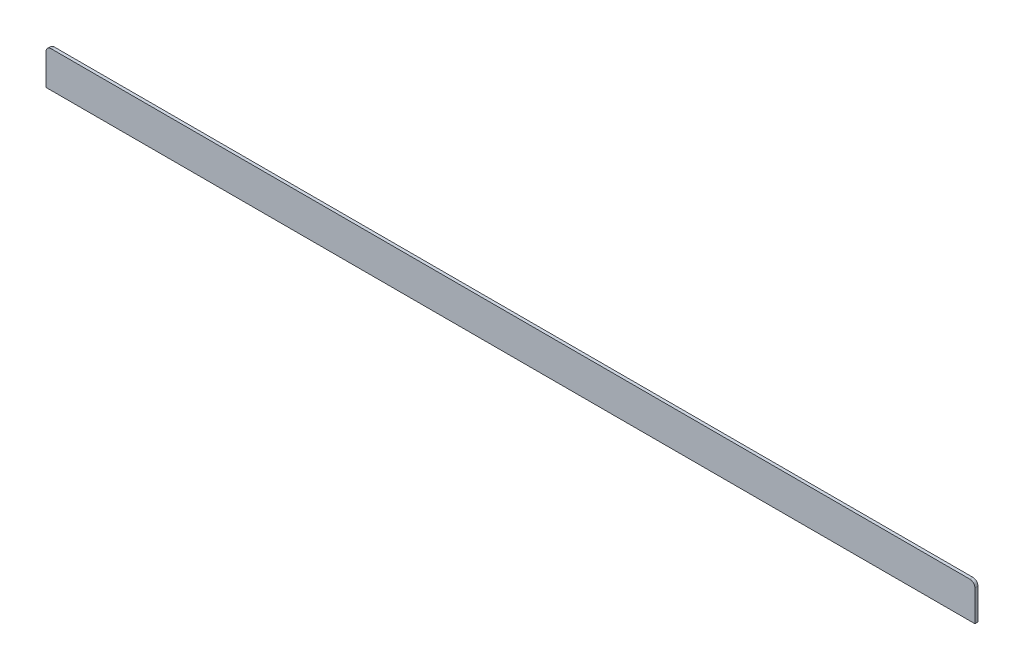
SolidWorks part; units mm, degrees
material "1023 碳钢板 (SS)"
ref_plane "前视基准面" through (0, 0, 0) normal (0, 0, 1) x (1, 0, 0)
ref_plane "上视基准面" through (0, 0, 0) normal (0, 1, 0) x (1, 0, 0)
ref_plane "右视基准面" through (0, 0, 0) normal (1, 0, 0) x (0, 0, -1)
sketch "草图1" plane through (0, 0, 0) normal (0, 0, 1) x (1, 0, 0)
  line L1 (-450, 17.5) -> (450, 17.5)
  line L2 (-450, 17.5) -> (-450, -17.5)
  line L3 (-450, -17.5) -> (450, -17.5)
  line L4 (450, 17.5) -> (450, -17.5)
  line L5 (-450, 17.5) -> (450, -17.5) construction
  line L6 (-450, -17.5) -> (450, 17.5) construction
  point P0 (0, 0)
  dimension "D1" = 900
  dimension "D2" = 35
extrude "凸台-拉伸1" add sketch "草图1" along normal blind 3
fillet "圆角1" radius 5 2 edges at (-450, 17.5, 1.5) (450, 17.5, 1.5)
